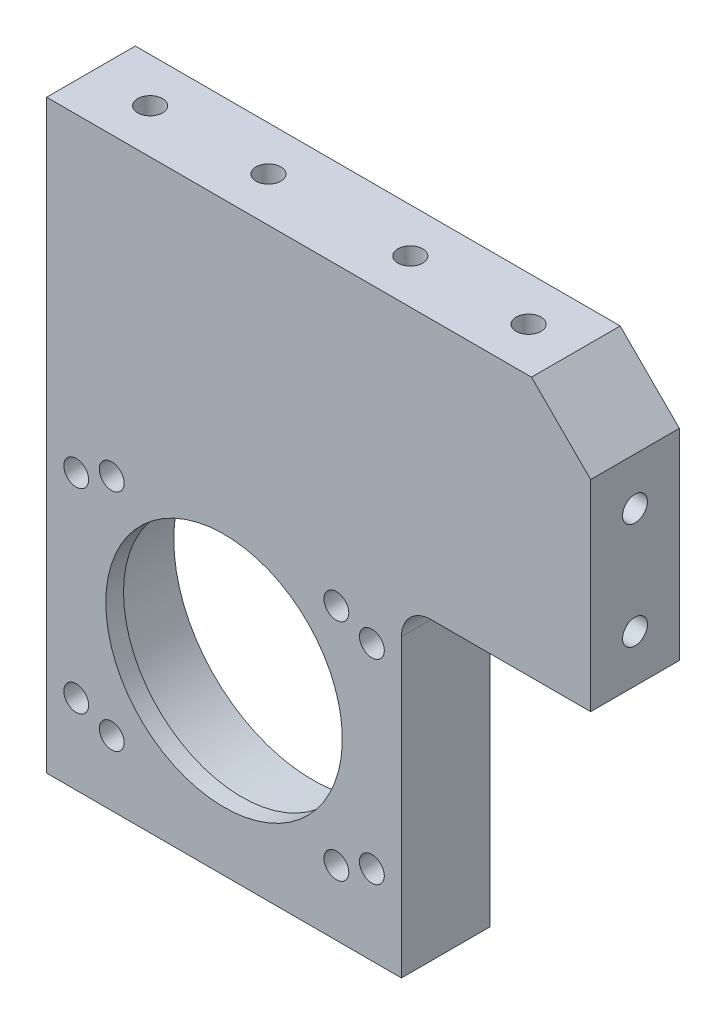
SolidWorks part; units mm, degrees
material "6061Al"
ref_plane "前视基准面" through (0, 0, 0) normal (0, 0, 1) x (1, 0, 0)
ref_plane "上视基准面" through (0, 0, 0) normal (0, 1, 0) x (1, 0, 0)
ref_plane "右视基准面" through (0, 0, 0) normal (1, 0, 0) x (0, 0, -1)
sketch "草图1" plane through (0, 0, 0) normal (0, 0, 1) x (1, 0, 0)
  line L1 (-55, -50) -> (55, -50)
  line L2 (-55, -50) -> (-55, 50)
  line L3 (-55, 50) -> (55, 50)
  line L4 (55, -50) -> (55, 50)
  line L5 (-55, -50) -> (55, 50) construction
  line L6 (-55, 50) -> (55, -50) construction
  point P0 (0, 0)
  dimension "D1" = 110
  dimension "D2" = 100
extrude "凸台-拉伸1" add sketch "草图1" along normal mid plane 15
sketch "草图10" plane through (0, 0, -7.5) normal (0, 0, 1) x (1, 0, 0)
  line L0 (55, 50) -> (-55, 50) construction
  line L1 (-55, 50) -> (-55, -50) construction
  circle A0 centre (-25, -20) radius 23.5
  dimension "D1" = 47
  dimension "D2" = 70
  dimension "D3" = 30
extrude "切除-拉伸1" cut sketch "草图10" along normal blind 12
sketch "草图12" plane through (0, 0, 4.5) normal (0, 0, -1) x (-1, 0, 0)
  circle A0 centre (25, -20) radius 20
  dimension "D1" = 40
extrude "切除-拉伸2" cut sketch "草图12" against normal through all
sketch "草图13" plane through (0, 0, 7.5) normal (0, 0, 1) x (1, 0, 0)
  line L0 (-55, -50) -> (55, -50) construction
  line L1 (5, -50) -> (55, -50)
  line L2 (5, -50) -> (5, 5)
  line L3 (5, 5) -> (55, 5)
  line L4 (55, -50) -> (55, 5)
  line L5 (55, -50) -> (55, 50) construction
  line L6 (-55, 50) -> (-55, -50) construction
  dimension "D1" = 60
  dimension "D2" = 55
extrude "切除-拉伸3" cut sketch "草图13" against normal through all
fillet "圆角1" radius 5 1 edges at (5, 5, 0)
hole_wizard "M5 螺纹孔1" positions "草图14" profile "草图15" tap size "M5" standard "ISO" end condition through all
sketch "草图14" plane through (0, 0, -7.5) normal (0, 0, -1) x (-1, 0, 0)
  circle A0 centre (25, -20) radius 20 construction
  point P13 (0, -3.5)
  point P16 (0, -36.5)
  point P19 (50, -36.5)
  point P22 (50, -3.5)
  dimension "D1" = 25
  dimension "D2" = 25
  dimension "D3" = 16.5
  dimension "D4" = 16.5
sketch "草图15" plane through (0, -3.5, -7.5) normal (1, 0, 0) x (0, 1, 0)
  line L0 (0, 0) -> (0, 15)
  line L1 (0, 15) -> (2.1, 15)
  line L2 (2.1, 15) -> (2.1, 0)
  line L5 (2.1, 0) -> (0, 0)
  line L11 (0, -6.35) -> (0, 107.95) construction
  dimension "通孔螺纹孔钻头直径" = 4.2
  dimension "通孔螺纹孔钻头深度" = 15
cosmetic thread "孔螺蚊线1" parameters "D2"=5
cosmetic thread "孔螺蚊线2" parameters "D2"=5
cosmetic thread "孔螺蚊线3" parameters "D2"=5
cosmetic thread "孔螺蚊线4" parameters "D2"=5
hole_wizard "M5 螺纹孔2" positions "草图16" profile "草图17" tap size "M5" standard "ISO" end condition through all
sketch "草图16" plane through (0, 0, 7.5) normal (0, 0, 1) x (1, 0, 0)
  circle A0 centre (-25, -20) radius 20 construction
  point P0 (-44, -1)
  point P3 (-44, -39)
  point P6 (-6, -39)
  point P9 (-6, -1)
sketch "草图17" plane through (-44, -1, 7.5) normal (1, 0, 0) x (0, -1, 0)
  line L0 (0, 0) -> (0, 15)
  line L1 (0, 15) -> (2.1, 15)
  line L2 (2.1, 15) -> (2.1, 0)
  line L5 (2.1, 0) -> (0, 0)
  line L11 (0, -6.35) -> (0, 107.95) construction
  dimension "通孔螺纹孔钻头直径" = 4.2
  dimension "通孔螺纹孔钻头深度" = 15
cosmetic thread "孔螺蚊线5" parameters "D2"=5
cosmetic thread "孔螺蚊线6" parameters "D2"=5
cosmetic thread "孔螺蚊线7" parameters "D2"=5
cosmetic thread "孔螺蚊线8" parameters "D2"=5
other "移动面1" face at (0, 50, 0) parameters "D1"=1
other "移动面2" face at (55, 27, 0) parameters "D1"=18
hole_wizard "M5 螺纹孔3" positions "草图18" profile "草图19" tap size "M5" standard "ISO"
sketch "草图18" plane through (0, 49, 0) normal (0, 1, 0) x (1, 0, 0)
  line L1 (-55, -7.5) -> (-55, 7.5) construction
  point P0 (19, 0)
  point P3 (-1, 0)
  point P6 (-25, 0)
  point P12 (-45, 0)
sketch "草图19" plane through (19, 49, 0) normal (1, 0, 0) x (0, 0, 1)
  line L0 (0, 0) -> (0, 13.6618)
  line L1 (0, 13.6618) -> (2.1, 12.4)
  line L2 (2.1, 12.4) -> (2.1, 0)
  line L5 (2.1, 0) -> (0, 0)
  line L10 (0, 13.6618) -> (-2.1, 12.4) construction
  line L11 (0, -6.35) -> (0, 107.95) construction
  dimension "螺纹孔钻头直径" = 4.2
  dimension "螺纹孔钻头深度" = 12.4
  dimension "导头角度" = 118
cosmetic thread "孔螺蚊线9" parameters "D1"=10, "D2"=5
cosmetic thread "孔螺蚊线10" parameters "D1"=10, "D2"=5
cosmetic thread "孔螺蚊线11" parameters "D1"=10, "D2"=5
cosmetic thread "孔螺蚊线14" parameters "D1"=10, "D2"=5
hole_wizard "M5 螺纹孔4" positions "草图20" profile "草图21" tap size "M5" standard "ISO"
sketch "草图20" plane through (37, 0, 0) normal (1, 0, 0) x (0, 0, -1)
  line L4 (-7.5, 49) -> (7.5, 49) construction
  point P0 (0, 13)
  point P3 (0, 31)
  dimension "D1" = 18
  dimension "D2" = 18
sketch "草图21" plane through (37, 13, 0) normal (0, 1, 0) x (0, 0, -1)
  line L0 (0, 0) -> (0, 13.6618)
  line L1 (0, 13.6618) -> (2.1, 12.4)
  line L2 (2.1, 12.4) -> (2.1, 0)
  line L5 (2.1, 0) -> (0, 0)
  line L10 (0, 13.6618) -> (-2.1, 12.4) construction
  line L11 (0, -6.35) -> (0, 107.95) construction
  dimension "螺纹孔钻头直径" = 4.2
  dimension "螺纹孔钻头深度" = 12.4
  dimension "导头角度" = 118
cosmetic thread "孔螺蚊线12" parameters "D1"=10, "D2"=5
cosmetic thread "孔螺蚊线13" parameters "D1"=10, "D2"=5
chamfer "倒角2" distance 10 angle 45 1 edges at (37, 49, 0)
move or copy body "实体-移动/复制1" [suppressed] bodies to move or copy 114 parameters "D1"=0, "D2"=0, "D3"=0
equation "\"D4@草图18\"=\"D2@草图18\""
equation "\"D1@草图16\"=\"D2@草图16\""
